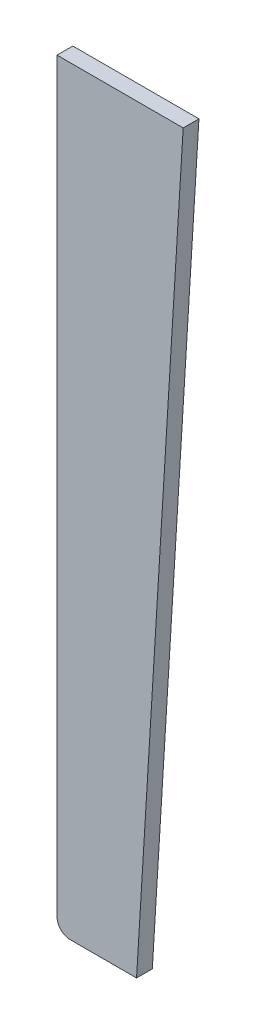
from build123d import *

# Parameters (mm, degrees)
BOSS_EXTRUDE1_DEPTH = 12


with BuildPart() as part:
    # Sketch1 → Boss-Extrude1 (new body)
    with BuildSketch(Plane.XY):
        with BuildLine():
            Line((0, 10), (0, 578))
            Line((0, 578), (96, 578))
            Line((96, 578), (60.5, 0))
            Line((60.5, 0), (10, 0))
            ThreePointArc((10, 0), (2.928932188, 2.928932188), (0, 10))
        make_face()
    extrude(amount=BOSS_EXTRUDE1_DEPTH)


solid = part.part
